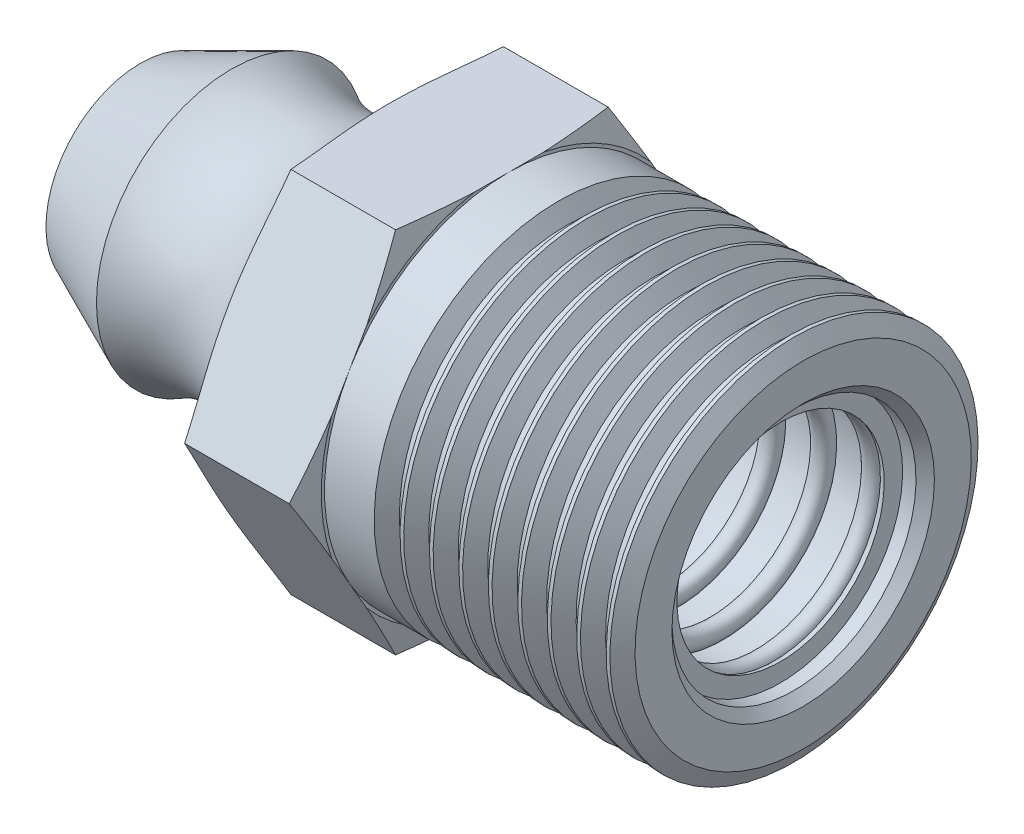
from build123d import *

# Parameters (mm, degrees)
SKETCH_1_R          = 0.25
SKETCH_2_R          = 10.539140362
CUT_EXTRUDE_1_DEPTH = 21.31501243


with BuildPart() as part:
    # 草图1 → 旋转1 (revolve)
    with BuildSketch(Plane.XY):
        with BuildLine():
            Line((-1.11345007, 3.314999999), (-10.5, 3.314999999))
            Line((-10.5, 3.314999999), (-11.5, 2.314999999))
            Line((-11.5, 2.314999999), (-16.471851993, 2.314999999))
            Line((-16.471851993, 2.314999999), (-17.89497877, 1.003746299))
            Line((-17.89497877, 1.003746299), (-18, 1.003746299))
            Line((-18, 1.003746299), (-18, 2.564999999))
            Line((-18, 2.564999999), (-15.529359549, 3.664999999))
            ThreePointArc((-15.529359549, 3.664999999), (-12.562954408, 3.565274985), (-11, 6.088502691))
            Line((-11, 6.088502691), (-8.267949192, 6.088502691))
            Line((-8.267949192, 6.088502691), (-8, 5.088502691))
            Line((-8, 5.088502691), (-8, 5))
            Line((-8, 5), (-6.65, 5))
            Line((-6.65, 5), (-6.4, 4.566987298))
            Line((-6.4, 4.566987298), (-6.2, 4.566987298))
            Line((-6.2, 4.566987298), (-5.95, 5))
            Line((-5.95, 5), (-5.85, 5))
            Line((-5.85, 5), (-5.6, 4.566987298))
            Line((-5.6, 4.566987298), (-5.4, 4.566987298))
            Line((-5.4, 4.566987298), (-5.15, 5))
            Line((-5.15, 5), (-5.05, 5))
            Line((-5.05, 5), (-4.8, 4.566987298))
            Line((-4.8, 4.566987298), (-4.6, 4.566987298))
            Line((-4.6, 4.566987298), (-4.35, 5))
            Line((-4.35, 5), (-4.25, 5))
            Line((-4.25, 5), (-4, 4.566987298))
            Line((-4, 4.566987298), (-3.8, 4.566987298))
            Line((-3.8, 4.566987298), (-3.55, 5))
            Line((-3.55, 5), (-3.45, 5))
            Line((-3.45, 5), (-3.2, 4.566987298))
            Line((-3.2, 4.566987298), (-3, 4.566987298))
            Line((-3, 4.566987298), (-2.75, 5))
            Line((-2.75, 5), (-2.65, 5))
            Line((-2.65, 5), (-2.4, 4.566987298))
            Line((-2.4, 4.566987298), (-2.2, 4.566987298))
            Line((-2.2, 4.566987298), (-1.95, 5))
            Line((-1.95, 5), (-1.85, 5))
            Line((-1.85, 5), (-1.6, 4.566987298))
            Line((-1.6, 4.566987298), (-1.4, 4.566987298))
            Line((-1.4, 4.566987298), (-1.15, 5))
            Line((-1.15, 5), (-1.05, 5))
            Line((-1.05, 5), (-0.8, 4.566987298))
            Line((-0.8, 4.566987298), (-0.6, 4.566987298))
            Line((-0.6, 4.566987298), (-0.35, 5))
            Line((-0.35, 5), (-0.25, 5))
            Line((-0.25, 5), (0, 4.566987298))
            Line((0, 4.566987298), (0, 3.564999999))
            Line((0, 3.564999999), (-0.25, 3.314999999))
            Line((-0.25, 3.314999999), (-0.61345007, 3.314999999))
            Line((-0.61345007, 3.314999999), (-0.61345007, 2.814999999))
            ThreePointArc((-0.61345007, 2.814999999), (-0.790226765, 2.888223303), (-0.86345007, 3.064999999))
            ThreePointArc((-0.86345007, 3.064999999), (-0.936673375, 3.241776694), (-1.11345007, 3.314999999))
        make_face()
        with BuildLine():
            ThreePointArc((-15.9, 0), (-17.15, 1.25), (-18.4, 0))
            Line((-18.4, 0), (-15.9, 0))
        make_face()
        with Locations((-15.888528375, 1.244283066)):
            Circle(SKETCH_1_R)
        with Locations((-14.657771147, 1.395401052)):
            Circle(SKETCH_1_R)
        with Locations((-13.427013919, 1.546519038)):
            Circle(SKETCH_1_R)
        with Locations((-12.19625669, 1.697637024)):
            Circle(SKETCH_1_R)
        with Locations((-10.965499462, 1.84875501)):
            Circle(SKETCH_1_R)
        with Locations((-9.734742234, 1.999872995)):
            Circle(SKETCH_1_R)
        with Locations((-8.503985006, 2.150990981)):
            Circle(SKETCH_1_R)
        with Locations((-7.273227778, 2.302108967)):
            Circle(SKETCH_1_R)
        with Locations((-6.04247055, 2.453226953)):
            Circle(SKETCH_1_R)
        with Locations((-4.811713322, 2.604344939)):
            Circle(SKETCH_1_R)
        with Locations((-3.580956094, 2.755462925)):
            Circle(SKETCH_1_R)
        with Locations((-2.350198866, 2.90658091)):
            Circle(SKETCH_1_R)
        with Locations((-1.119441638, 3.057698896)):
            Circle(SKETCH_1_R)
    revolve(axis=Axis((0, 0, 0), (-1, 0, 0)))

    # 草图2 → 切除-拉伸1 (cut, through all)
    with BuildSketch(Plane(origin=(0, 0, 0), x_dir=(0, 0, -1), z_dir=(1, 0, 0))):
        Circle(SKETCH_2_R)
        Polygon((5.773502692, 0), (2.886751346, 5), (-2.886751346, 5), (-5.773502692, 0), (-2.886751346, -5), (2.886751346, -5), align=None, mode=Mode.SUBTRACT)
    extrude(amount=-CUT_EXTRUDE_1_DEPTH, mode=Mode.SUBTRACT)


solid = part.part
